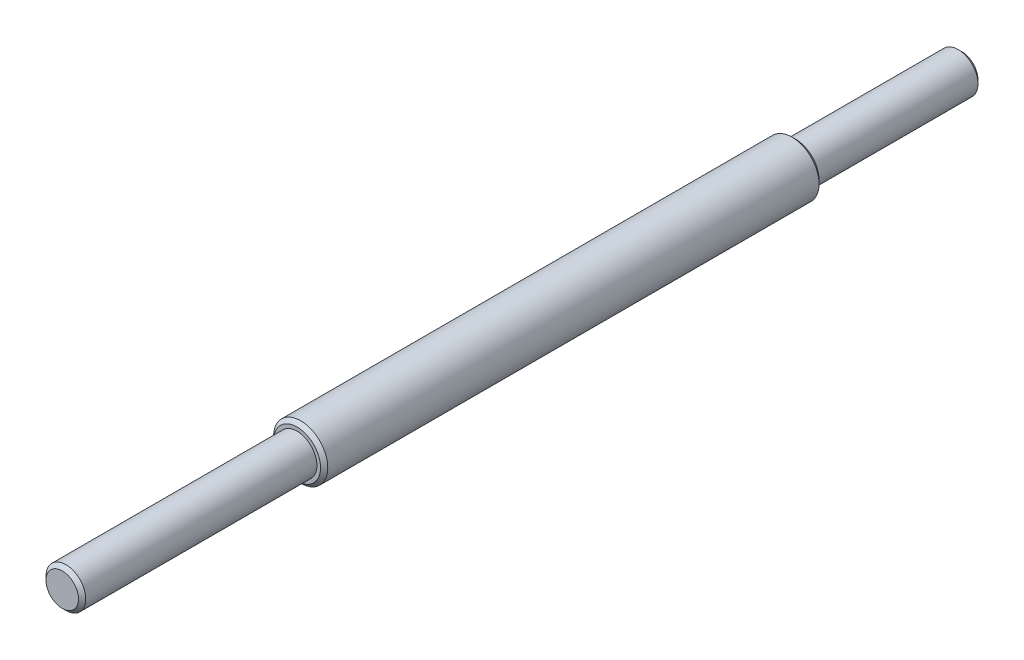
from build123d import *

# Parameters (mm, degrees)
SKETCH1_R           = 7.5
BOSS_EXTRUDE1_DEPTH = 138
SKETCH2_R           = 5.5
BOSS_EXTRUDE2_DEPTH = 20
SKETCH3_R           = 5.5
BOSS_EXTRUDE3_DEPTH = 45
CHAMFER1_SIZE       = 1
BOSS_EXTRUDE4_START = 46
SKETCH4_R           = 5.5
BOSS_EXTRUDE4_DEPTH = 46
CHAMFER2_SIZE       = 1


with BuildPart() as part:
    # Sketch1 → Boss-Extrude1 (new body)
    with BuildSketch(Plane.XY):
        Circle(SKETCH1_R)
    extrude(amount=BOSS_EXTRUDE1_DEPTH)

    # Sketch2 → Boss-Extrude2 (add)
    with BuildSketch(Plane.XY.offset(138)):
        Circle(SKETCH2_R)
    extrude(amount=BOSS_EXTRUDE2_DEPTH)

    # Sketch3 → Boss-Extrude3 (add)
    with BuildSketch(Plane.XY.offset(158)):
        Circle(SKETCH3_R)
    extrude(amount=BOSS_EXTRUDE3_DEPTH)

    # Chamfer1
    chamfer1_edges = [part.edges().sort_by_distance(p)[0] for p in [
        (-7.5, 0, 0),
        (-7.5, 0, 138),
        (-5.5, 0, 203),
    ]]
    chamfer(chamfer1_edges, length=CHAMFER1_SIZE)

    # Sketch4 → Boss-Extrude4 (add)
    with BuildSketch(Plane(origin=(0, 0, 0), x_dir=(-1, 0, 0), z_dir=(0, 0, -1)).offset(BOSS_EXTRUDE4_START)):
        with Locations(Location((0, 0, 0), (0, 0, 180))):
            Circle(SKETCH4_R)
    extrude(amount=-BOSS_EXTRUDE4_DEPTH)

    # Chamfer2
    chamfer2_edges = [part.edges().sort_by_distance(p)[0] for p in [
        (-5.5, 0, -46),
    ]]
    chamfer(chamfer2_edges, length=CHAMFER2_SIZE)


solid = part.part
